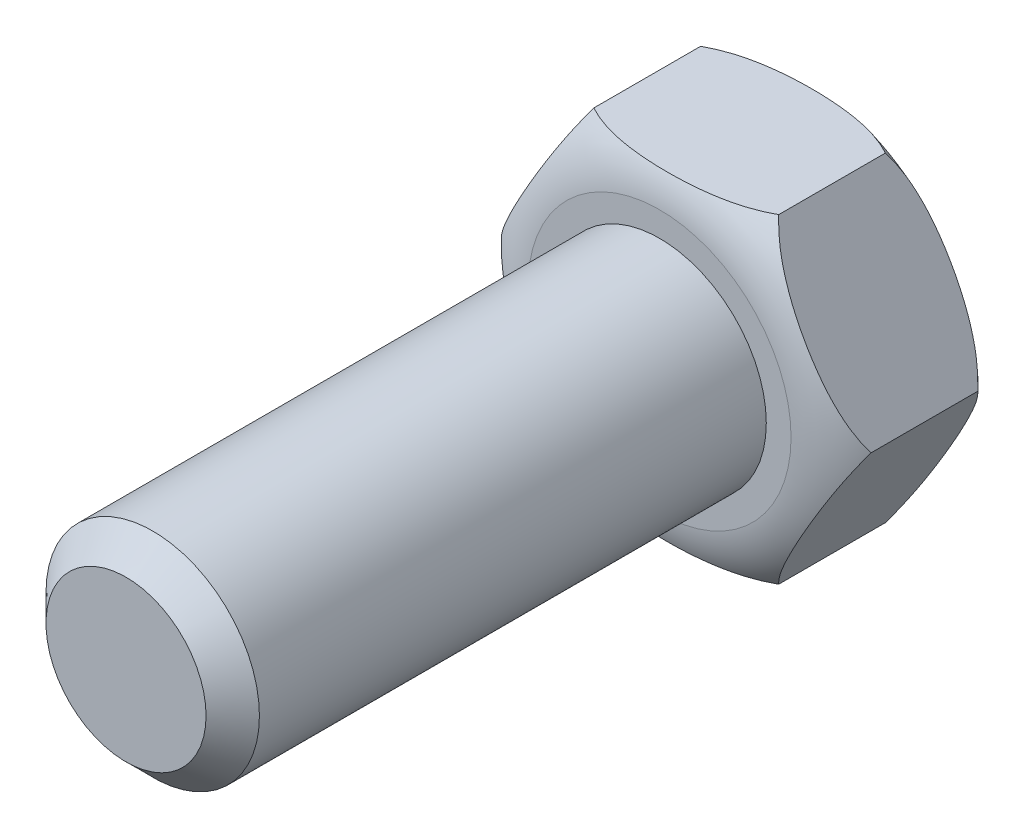
SolidWorks part; units mm, degrees
ref_plane "Front" through (0, 0, 0) normal (0, 0, 1) x (1, 0, 0)
ref_plane "Top" through (0, 0, 0) normal (0, 1, 0) x (1, 0, 0)
ref_plane "Right" through (0, 0, 0) normal (1, 0, 0) x (0, 0, -1)
sketch "Sketch1" plane through (0, 0, 0) normal (0, 0, 1) x (1, 0, 0)
  line L1 (6.9282, 0) -> (3.4641, 6)
  line L2 (3.4641, 6) -> (-3.4641, 6)
  line L3 (-3.4641, 6) -> (-6.9282, 0)
  line L4 (-6.9282, 0) -> (-3.4641, -6)
  line L5 (-3.4641, -6) -> (3.4641, -6)
  line L6 (3.4641, -6) -> (6.9282, 0)
  circle A0 centre (0, 0) radius 6 construction
  dimension "D1" = 12
extrude "Boss-Extrude1" add sketch "Sketch1" along normal blind 6
sketch "Sketch2" plane through (0, 0, 6) normal (0, 0, 1) x (1, 0, 0)
  circle A0 centre (0, 0) radius 4
  dimension "D1" = 8
extrude "Boss-Extrude2" add sketch "Sketch2" along normal blind 20
chamfer "Chamfer1" distance 1 angle 45 1 edges at (4, 0, 26)
sketch "Sketch3" plane through (0, 0, 0) normal (0, 1, 0) x (1, 0, 0)
  line L0 (-4.9282, 0) -> (-4.9282, -1)
  line L1 (-9.3113, -1) -> (-4.9282, -1)
  line L2 (-9.3113, -5) -> (-6.9282, -5)
  line L3 (-6.9282, -6) -> (-6.9282, 0) construction
  line L4 (-3.4641, 0) -> (-6.9282, 0) construction
  line L5 (-3.4641, -6) -> (-6.9282, -6) construction
  line L6 (-9.3113, -1) -> (-8.8538, 0.8513)
  line L7 (-8.8538, 0.8513) -> (-4.9282, 0)
  line L8 (-9.3113, -5) -> (-8.016, -6.7449)
  line L9 (-8.016, -6.7449) -> (-4.9282, -6)
  line L10 (0, 0) -> (0, 4.959) construction
  arc A0 (-4.9282, 0) -> (-6.9282, -1) centre (-4.6832, -2.99) ccw
  arc A1 (-6.9282, -5) -> (-4.9282, -6) centre (-4.6832, -3.01) ccw
  dimension "D4" = 3
  dimension "D5" = 3
  dimension "D1" = 2
  dimension "D2" = 1
  dimension "D3" = 1
revolve "Cut-Revolve1" cut sketch "Sketch3" angle 360 about L10
scale "Scale 1" bodies to scale 103 scale about centroid uniform scaling yes scale factor 1.875
